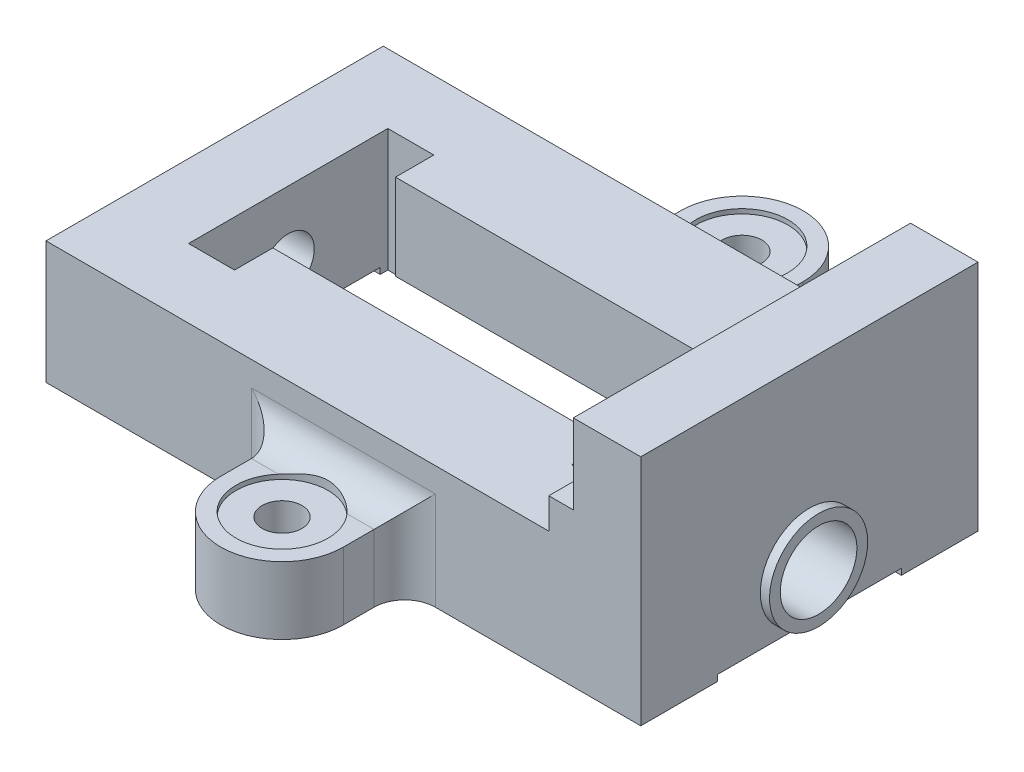
from build123d import *

# Parameters (mm, degrees)
BOSS_EXTRUDE1_DEPTH     = 55
SKETCH2_W               = 60
SKETCH2_H               = 2
CUT_EXTRUDE1_DEPTH      = 212
SKETCH3_R               = 16
BOSS_EXTRUDE2_DEPTH     = 3
SKETCH4_R               = 12.5
CUT_EXTRUDE2_DEPTH      = 56
SKETCH5_R               = 12.5
BOSS_EXTRUDE3_DEPTH     = 3
SKETCH6_R               = 8.5
CUT_EXTRUDE3_DEPTH      = 66
CUT_EXTRUDE4_DEPTH      = 28
SKETCH9_R               = 6.5
BOSS_EXTRUDE4_DEPTH     = 22
FILLET1_R               = 10
CUT_EXTRUDE5_DEPTH      = 15.5
CUT_EXTRUDE5_DEPTH_BACK = 1.5
SKETCH10_R              = 15
SKETCH12_W              = 110
SKETCH12_H              = 12.5
SKETCH12_H_2            = 2.5
SKETCH12_H_3            = 10
SKETCH12_W_2            = 15
CUT_EXTRUDE7_DEPTH      = 12
SKETCH13_R              = 3
CUT_EXTRUDE8_DEPTH      = 10


with BuildPart() as part:
    # Sketch1 → Boss-Extrude1 (new, symmetric)
    with BuildSketch(Plane.XY):
        Polygon((0, 0), (194, 0), (194, 29.332947361), (194, 76), (172, 76), (172, 50), (164, 50), (164, 40), (0, 40), align=None)
    extrude(amount=BOSS_EXTRUDE1_DEPTH, both=True)

    # Sketch2 → Cut-Extrude1 (cut)
    with BuildSketch(Plane(origin=(194, 0, 0), x_dir=(0, 0, -1), z_dir=(1, 0, 0))):
        with Locations((0, 1)):
            Rectangle(SKETCH2_W, SKETCH2_H)
    extrude(amount=-CUT_EXTRUDE1_DEPTH, mode=Mode.SUBTRACT)

    # Sketch3 → Boss-Extrude2 (add)
    with BuildSketch(Plane(origin=(194, 0, 0), x_dir=(0, 0, -1), z_dir=(1, 0, 0))):
        with Locations(Location((0, 18, 0), (0, 0, 270))):
            Circle(SKETCH3_R)
    extrude(amount=BOSS_EXTRUDE2_DEPTH)

    # Sketch4 → Cut-Extrude2 (cut)
    with BuildSketch(Plane(origin=(197, 0, 0), x_dir=(0, 0, -1), z_dir=(1, 0, 0))):
        with Locations((0, 18)):
            Circle(SKETCH4_R)
    extrude(amount=-CUT_EXTRUDE2_DEPTH, mode=Mode.SUBTRACT)

    # Sketch5 → Boss-Extrude3 (add)
    with BuildSketch(Plane.ZY):
        with Locations(Location((0, 18, 0), (0, 0, 180))):
            Circle(SKETCH5_R)
    extrude(amount=BOSS_EXTRUDE3_DEPTH)

    # Sketch6 → Cut-Extrude3 (cut)
    with BuildSketch(Plane.ZY.offset(3)):
        with Locations(Location((0, 18, 0), (0, 0, 270))):
            Circle(SKETCH6_R)
    extrude(amount=-CUT_EXTRUDE3_DEPTH, mode=Mode.SUBTRACT)

    # Sketch7 → Cut-Extrude4 (cut)
    with BuildSketch(Plane(origin=(0, 40, 0), x_dir=(1, 0, 0), z_dir=(0, 1, 0))):
        Polygon((164, 32.5), (149, 32.5), (149, 20), (39, 20), (39, 32.5), (24, 32.5), (24, -32.5), (39, -32.5), (39, -20), (149, -20), (149, -32.5), (164, -32.5), align=None)
    extrude(amount=-CUT_EXTRUDE4_DEPTH, mode=Mode.SUBTRACT)

    # Sketch9 → Boss-Extrude4 (add)
    with BuildSketch(Plane.XZ):
        with BuildLine():
            Line((117, 75), (117, 65))
            ThreePointArc((117, 65), (119.928932188, 57.928932188), (127, 55))
            Line((127, 55), (67, 55))
            ThreePointArc((67, 55), (74.071067812, 57.928932188), (77, 65))
            Line((77, 65), (77, 75))
            ThreePointArc((77, 75), (97, 95), (117, 75))
        make_face()
        with Locations(Location((97, 75, 0), (0, 0, 270))):
            Circle(SKETCH9_R, mode=Mode.SUBTRACT)
    extrude(amount=-BOSS_EXTRUDE4_DEPTH)

    # Fillet1
    fillet1_edges = [part.edges().sort_by_distance(p)[0] for p in [
        (97, 22, 55),
    ]]
    fillet(fillet1_edges, radius=FILLET1_R)

    # Sketch10 → Cut-Extrude5 (cut, two sides: drawn at the far end of the back side and taken through both)
    with BuildSketch(Plane(origin=(0, 22, 0), x_dir=(1, 0, 0), z_dir=(0, 1, 0)).offset(-CUT_EXTRUDE5_DEPTH_BACK)):
        with Locations(Location((97, -75, 0), (0, 0, 138.189685104))):
            Circle(SKETCH10_R)
    extrude(amount=CUT_EXTRUDE5_DEPTH + CUT_EXTRUDE5_DEPTH_BACK, mode=Mode.SUBTRACT)

    # Mirror17: part across plane


with BuildPart() as part_1:
    add(part.part)
    add(part.part.mirror(Plane.XY))

    # Sketch12 → Cut-Extrude7 (cut)
    with BuildSketch(Plane.XZ):
        Polygon((149, 20), (39, 20), (39, 32.5), (24, 32.5), (24, -30), (39, -30), (39, -20), (149, -20), (149, -30), (164, -30), (164, 32.5), (149, 32.5), align=None)
        with Locations((94, 26.25)):
            Rectangle(SKETCH12_W, SKETCH12_H)
        with Locations((94, -31.25)):
            Rectangle(SKETCH12_W, SKETCH12_H_2)
        with Locations((94, -25)):
            Rectangle(SKETCH12_W, SKETCH12_H_3)
        with Locations((31.5, -31.25)):
            Rectangle(SKETCH12_W_2, SKETCH12_H_2)
        with Locations((156.5, -31.25)):
            Rectangle(SKETCH12_W_2, SKETCH12_H_2)
    extrude(amount=-CUT_EXTRUDE7_DEPTH, mode=Mode.SUBTRACT)

    # Sketch13 → Cut-Extrude8 (cut)
    with BuildSketch(Plane.ZY.offset(-172)):
        with Locations(Location((38, 63, 0), (0, 0, 270))):
            Circle(SKETCH13_R)
        with Locations(Location((-38, 63, 0), (0, 0, 90))):
            Circle(SKETCH13_R)
    extrude(amount=-CUT_EXTRUDE8_DEPTH, mode=Mode.SUBTRACT)


solid = part_1.part
